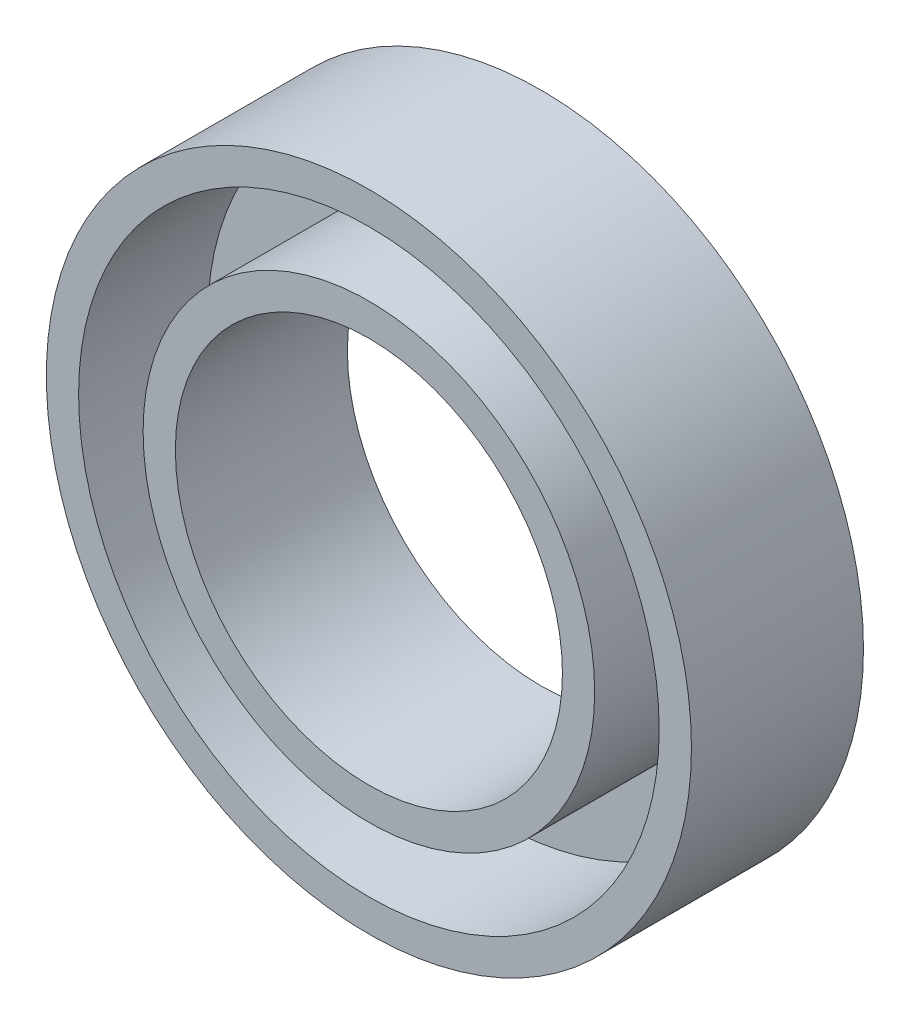
SolidWorks part; units mm, degrees
ref_plane "Front Plane" through (0, 0, 0) normal (0, 0, 1) x (1, 0, 0)
ref_plane "Top Plane" through (0, 0, 0) normal (0, 1, 0) x (1, 0, 0)
ref_plane "Right Plane" through (0, 0, 0) normal (1, 0, 0) x (0, 0, -1)
sketch "Sketch1" plane through (0, 0, 0) normal (0, 0, 1) x (1, 0, 0)
  circle A0 centre (0, 0) radius 15
  circle A1 centre (0, 0) radius 9
  dimension "D1" = 30
  dimension "D2" = 18
extrude "Boss-Extrude1" add sketch "Sketch1" along normal blind 8
sketch "Sketch2" plane through (0, 0, 8) normal (0, 0, 1) x (1, 0, 0)
  circle A2 centre (0, 0) radius 13.5
  circle A3 centre (0, 0) radius 13.5
  circle A5 centre (0, 0) radius 10.5
  circle A6 centre (0, 0) radius 10.5
  dimension "D1" = 1.5
  dimension "D2" = 1.5
extrude "Cut-Extrude1" cut sketch "Sketch2" against normal offset from surface (6 mm away) 2 up to face at (15, 0, 0)
